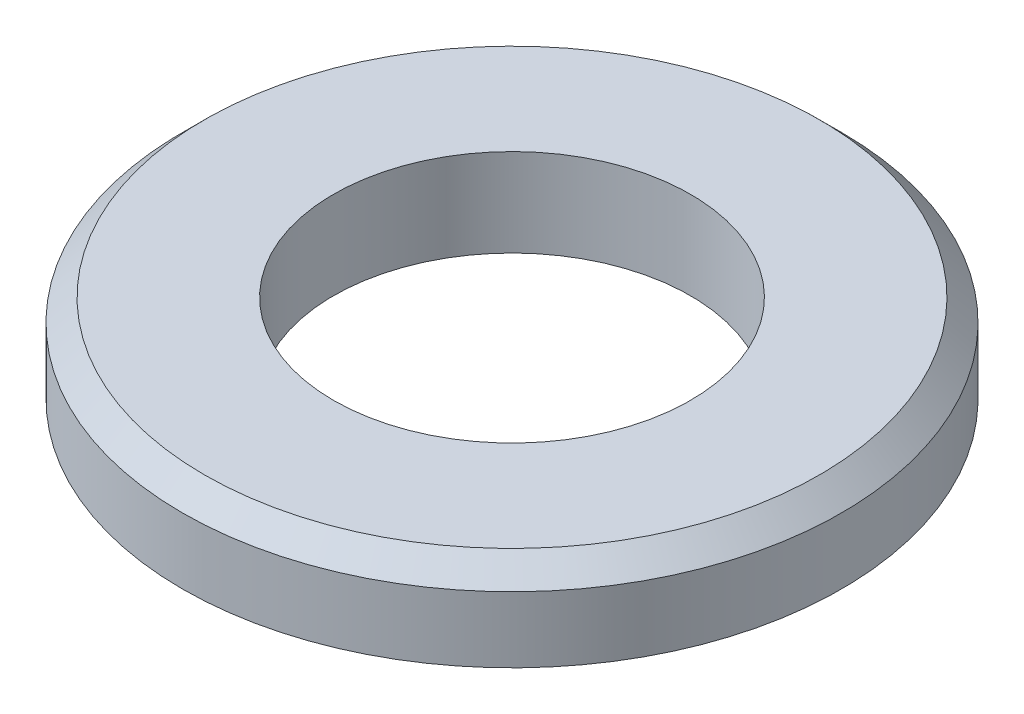
from build123d import *

# Parameters (mm, degrees)
SKETCH1_R           = 6
SKETCH1_R_2         = 3.25
BOSS_EXTRUDE1_DEPTH = 1.6
CHAMFER1_SIZE       = 0.4


with BuildPart() as part:
    # Sketch1 → Boss-Extrude1 (new body)
    with BuildSketch(Plane(origin=(0, 0, 0), x_dir=(1, 0, 0), z_dir=(0, 1, 0))):
        with Locations(Location((0, 0, 0), (0, 0, 270))):
            Circle(SKETCH1_R)
        with Locations(Location((0, 0, 0), (0, 0, 270))):
            Circle(SKETCH1_R_2, mode=Mode.SUBTRACT)
    extrude(amount=BOSS_EXTRUDE1_DEPTH)

    # Chamfer1
    chamfer1_edges = [part.edges().sort_by_distance(p)[0] for p in [
        (0, 1.6, -6),
    ]]
    chamfer(chamfer1_edges, length=CHAMFER1_SIZE)


solid = part.part
